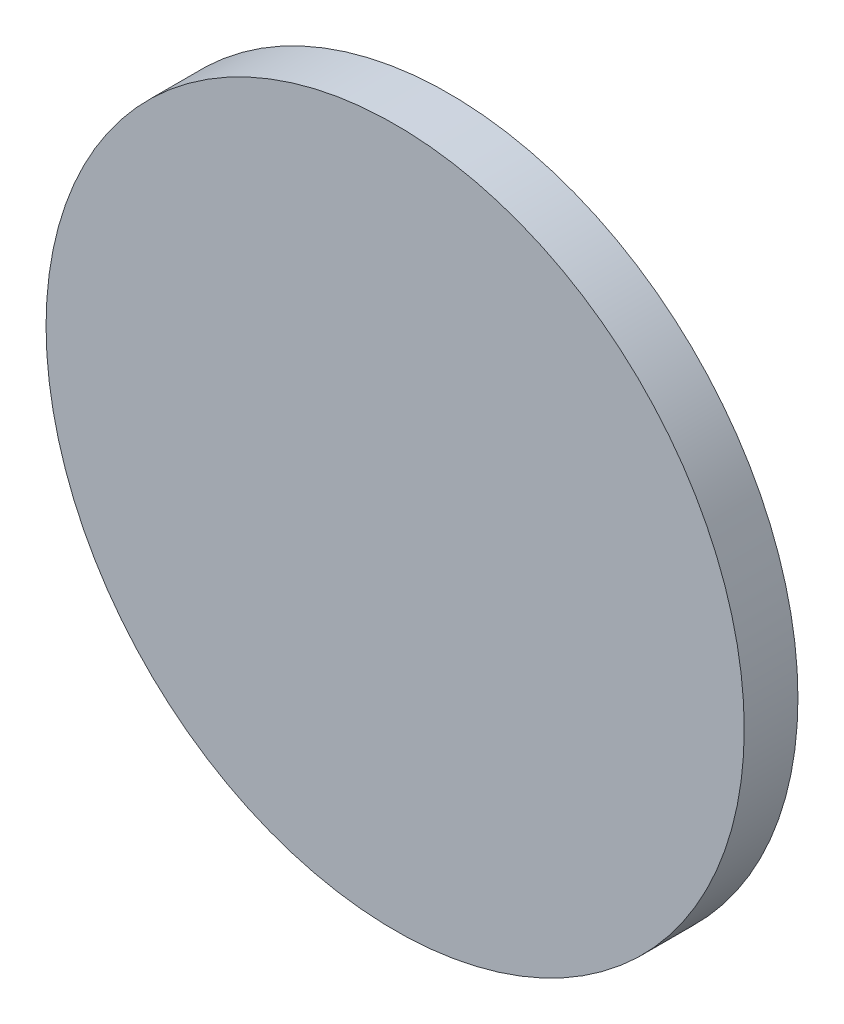
from build123d import *

# Parameters (mm, degrees)
SKETCH1_R           = 65
BOSS_EXTRUDE1_DEPTH = 10


with BuildPart() as part:
    # Sketch1 → Boss-Extrude1 (new body)
    with BuildSketch(Plane.XY):
        Circle(SKETCH1_R)
    extrude(amount=BOSS_EXTRUDE1_DEPTH)


solid = part.part
